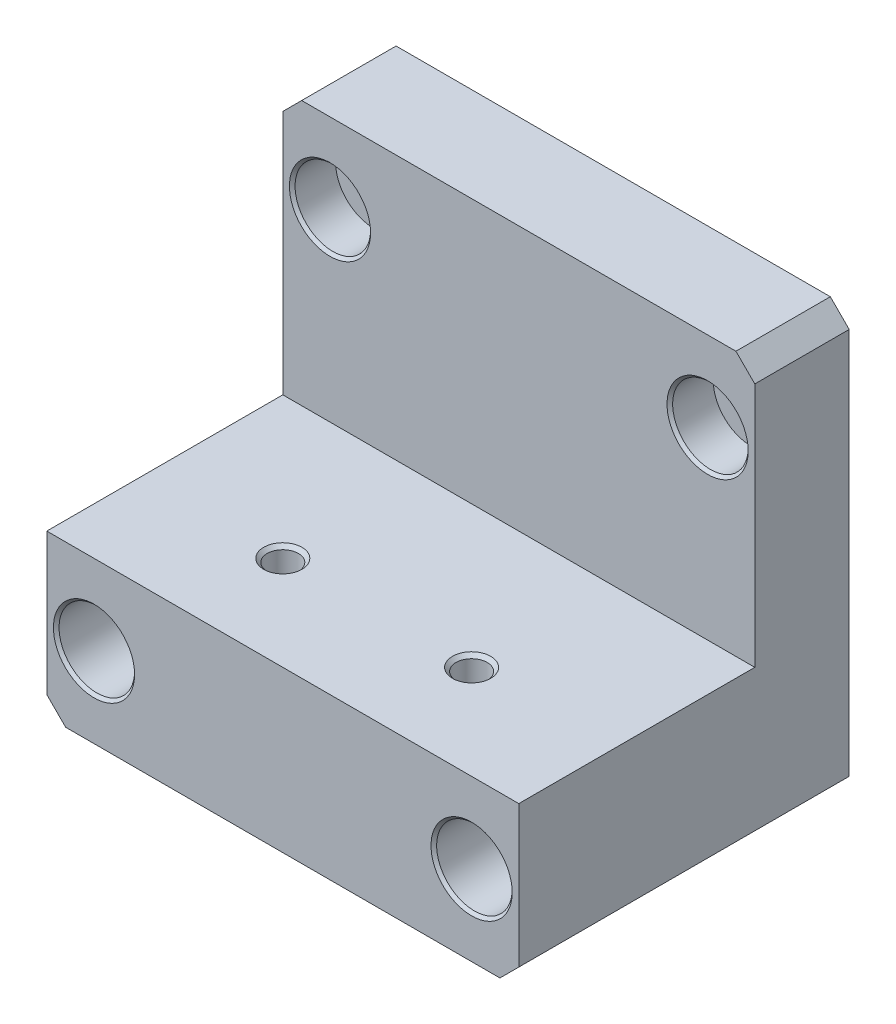
from build123d import *

# Parameters (mm, degrees)
SKETCH_1_W                   = 50
SKETCH_1_H                   = 45
EXTRUDE_1_DEPTH              = 10
SKETCH_6_W                   = 50
SKETCH_6_H                   = 17
EXTRUDE_2_DEPTH              = 25
CHAMFER_1_SIZE               = 2
HOLE_WIZARD_1_AT_2_COUNT     = 2
HOLE_WIZARD_1_AT_2_PITCH     = 40
HOLE_WIZARD_2_AT_2_COUNT     = 2
HOLE_WIZARD_2_AT_2_PITCH     = 40
HOLE_WIZARD_M4_1_D           = 3.3
HOLE_WIZARD_M4_1_CSINK_D     = 4.05
HOLE_WIZARD_M4_1_CSINK_ANGLE = 90


with BuildPart() as part:
    # 草图1 → 凸台-拉伸1 (new body)
    with BuildSketch(Plane.XY):
        with Locations((-25, 22.5)):
            Rectangle(SKETCH_1_W, SKETCH_1_H)
    extrude(amount=EXTRUDE_1_DEPTH)

    # 草图6 → 凸台-拉伸2 (add)
    with BuildSketch(Plane.XY.offset(10)):
        with Locations((-25, 8.5)):
            Rectangle(SKETCH_6_W, SKETCH_6_H)
    extrude(amount=EXTRUDE_2_DEPTH)

    # 倒角1
    chamfer_1_edges = [part.edges().sort_by_distance(p)[0] for p in [
        (0, 0, 17.5),
        (-50, 0, 17.5),
        (-50, 45, 5),
        (0, 45, 5),
    ]]
    chamfer(chamfer_1_edges, length=CHAMFER_1_SIZE)

    # 草图4 → 打孔尺寸(%根据)内六角圆柱头螺钉的类型1 (revolve, cut)
    with BuildSketch(Plane(origin=(-45, 36.5, 10), x_dir=(0, -1, 0), z_dir=(1, 0, 0))):
        Polygon((0, 0), (0, 11.291850331), (2.15, 10), (2.15, 4.6), (4, 4.6), (4, 0.3), (4.3, 0), align=None)
    hole_wizard_1 = revolve(axis=Axis((-45, 36.5, 16.35), (0, 0, -1)), mode=Mode.SUBTRACT)

    # 打孔尺寸(%根据)内六角圆柱头螺钉的类型1 at 2: 打孔尺寸(%根据)内六角圆柱头螺钉的类型1 ×2
    with Locations(*[(i * HOLE_WIZARD_1_AT_2_PITCH, 0, 0) for i in range(1, HOLE_WIZARD_1_AT_2_COUNT)]):
        add(hole_wizard_1, mode=Mode.SUBTRACT)

    # 草图8 → 打孔尺寸(%根据)内六角圆柱头螺钉的类型2 (revolve, cut)
    with BuildSketch(Plane(origin=(-45, 8.5, 35), x_dir=(0, -1, 0), z_dir=(1, 0, 0))):
        Polygon((0, 0), (0, 35), (2.15, 35), (2.15, 25), (4, 25), (4, 0.3), (4.3, 0), align=None)
    hole_wizard_2 = revolve(axis=Axis((-45, 8.5, 41.35), (0, 0, -1)), mode=Mode.SUBTRACT)

    # 打孔尺寸(%根据)内六角圆柱头螺钉的类型2 at 2: 打孔尺寸(%根据)内六角圆柱头螺钉的类型2 ×2
    with Locations(*[(i * HOLE_WIZARD_2_AT_2_PITCH, 0, 0) for i in range(1, HOLE_WIZARD_2_AT_2_COUNT)]):
        add(hole_wizard_2, mode=Mode.SUBTRACT)

    # M4 螺纹孔1 (through all)
    with Locations(Plane(origin=(0, 17, 0), x_dir=(1, 0, 0), z_dir=(0, 1, 0))):
        with Locations((-35, -25), (-15, -25)):
            CounterSinkHole(HOLE_WIZARD_M4_1_D / 2, HOLE_WIZARD_M4_1_CSINK_D / 2, counter_sink_angle=HOLE_WIZARD_M4_1_CSINK_ANGLE)


solid = part.part
